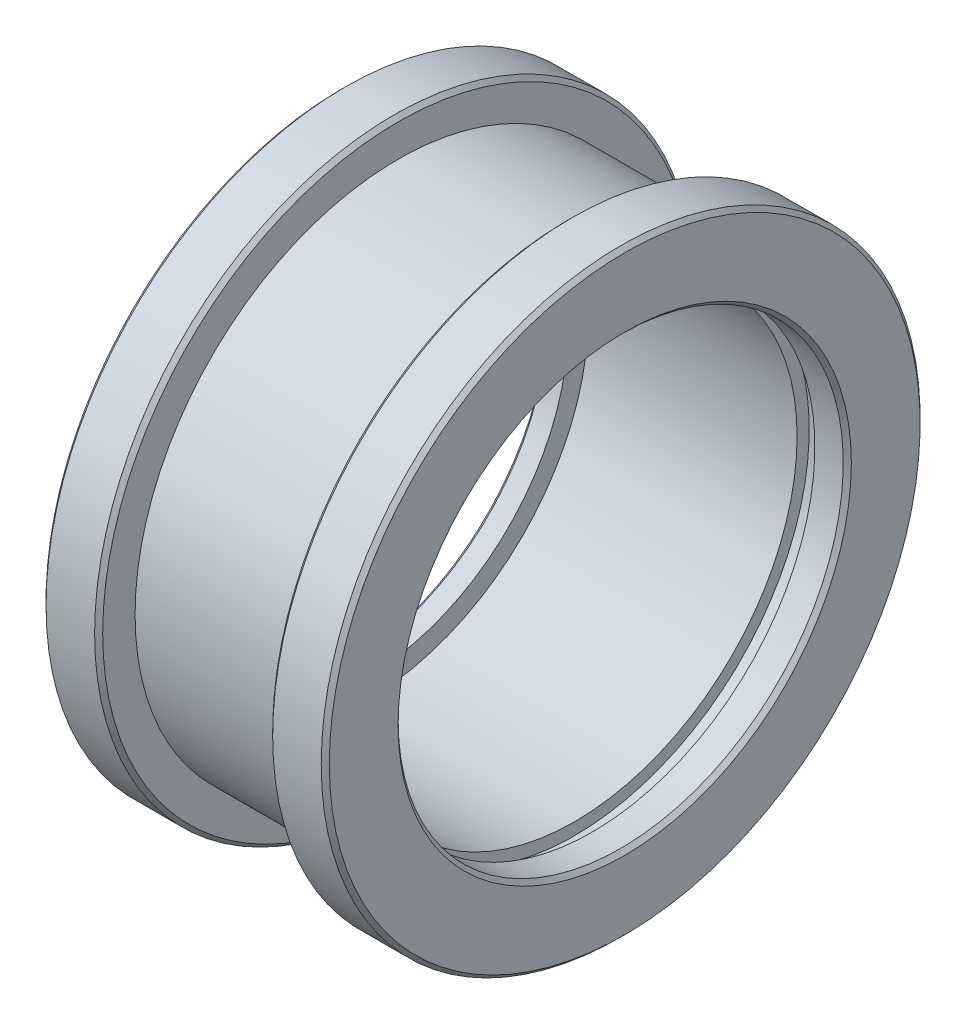
SolidWorks part; units mm, degrees
ref_plane "前视基准面" through (0, 0, 0) normal (0, 0, 1) x (1, 0, 0)
ref_plane "上视基准面" through (0, 0, 0) normal (0, 1, 0) x (1, 0, 0)
ref_plane "右视基准面" through (0, 0, 0) normal (1, 0, 0) x (0, 0, -1)
sketch "草图1" plane through (0, 0, 0) normal (0, 0, 1) x (1, 0, 0)
  line L0 (-17.5, 0) -> (17.5, 0)
  line L1 (17.5, 37) -> (10.5, 37)
  line L2 (10.5, 37) -> (10.5, 32.5)
  line L3 (10.5, 32.5) -> (-10.5, 32.5)
  line L4 (-10.5, 32.5) -> (-10.5, 37)
  line L5 (-10.5, 37) -> (-17.5, 37)
  line L6 (-17.5, 37) -> (-17.5, 0)
  line L7 (17.5, 0) -> (17.5, 37)
  line L8 (0, 0) -> (0, 151.8973) construction
  dimension "D1" = 35
  dimension "D2" = 37
  dimension "D3" = 32.5
  dimension "D4" = 21
revolve "旋转1" add sketch "草图1" angle 360 about L0
sketch "草图2" plane through (17.5, 0, 0) normal (1, 0, 0) x (0, 0, -1)
  circle A0 centre (0, 0) radius 27.5
  dimension "D1" = 55
extrude "切除-拉伸1" cut sketch "草图2" against normal blind 32
sketch "草图4" plane through (-14.5, 0, 0) normal (1, 0, 0) x (0, 0, -1)
  circle A0 centre (0, 0) radius 25
  dimension "D1" = 50
extrude "切除-拉伸2" cut sketch "草图4" against normal blind 30
chamfer "倒角1" distance 0.5 angle 45 6 edges at (10.5, 0, 37) (-10.5, 0, 37) (-17.5, 0, -25) (17.5, 0, -27.5) (-17.5, 0, 37) (17.5, 0, 37)
sketch "草图5" plane through (0, 0, 0) normal (0, 1, 0) x (1, 0, 0)
  line L0 (17, 27.5) -> (-14.5, 27.5) construction
  line L1 (11.3, 27.5) -> (13.5, 27.5)
  line L2 (11.3, 27.5) -> (11.3, 29)
  line L3 (11.3, 29) -> (13.5, 29)
  line L4 (13.5, 27.5) -> (13.5, 29)
  line L5 (17.5, -36.5) -> (17.5, 36.5) construction
  line L6 (0, 0) -> (30.4268, 0) construction
  dimension "D1" = 1.5
  dimension "D2" = 2.2
  dimension "D3" = 4
revolve "切除-旋转1" cut sketch "草图5" angle 360 about L6
